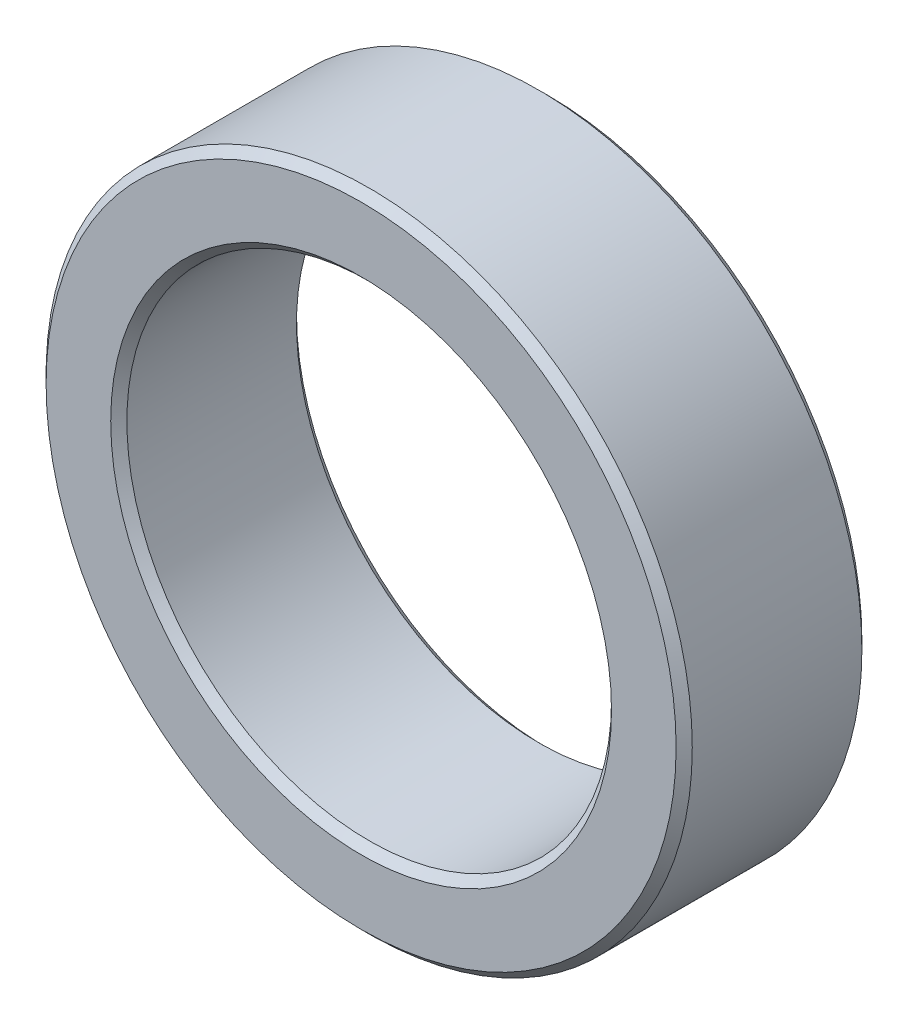
from build123d import *

# Parameters (mm, degrees)
SKETCH1_R           = 40
SKETCH1_R_2         = 30
BOSS_EXTRUDE1_DEPTH = 11.5
CHAMFER1_SIZE       = 1


with BuildPart() as part:
    # Sketch1 → Boss-Extrude1 (new, symmetric)
    with BuildSketch(Plane.XY):
        Circle(SKETCH1_R)
        Circle(SKETCH1_R_2, mode=Mode.SUBTRACT)
    extrude(amount=BOSS_EXTRUDE1_DEPTH, both=True)

    # Chamfer1
    chamfer1_edges = [part.edges().sort_by_distance(p)[0] for p in [
        (-40, 0, -11.5),
        (-40, 0, 11.5),
        (-30, 0, -11.5),
        (-30, 0, 11.5),
    ]]
    chamfer(chamfer1_edges, length=CHAMFER1_SIZE)


solid = part.part
